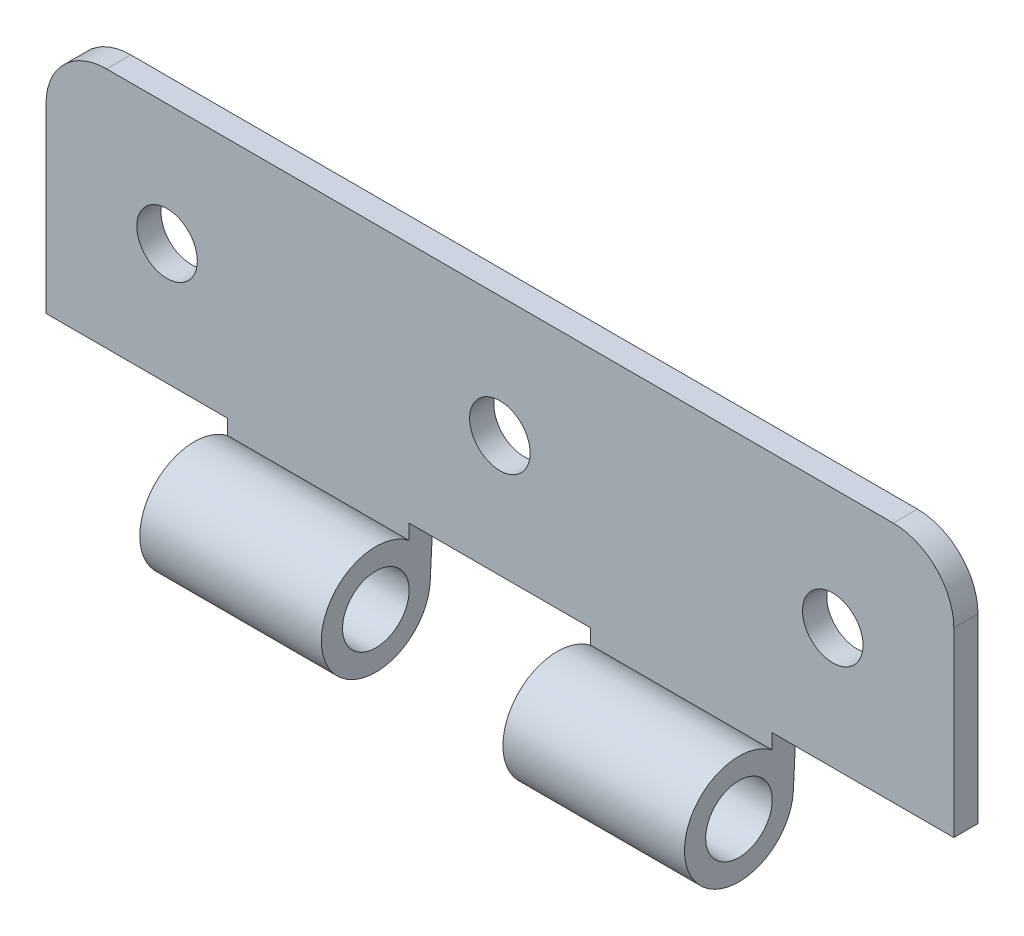
from build123d import *

# Parameters (mm, degrees)
SKETCH1_W           = 75
SKETCH1_H           = 20
SKETCH1_R           = 2.5
BOSS_EXTRUDE1_DEPTH = 2
BOSS_EXTRUDE2_START = -15
BOSS_EXTRUDE2_DEPTH = 15
LPATTERN1_COUNT     = 2
LPATTERN1_PITCH     = 30
FILLET1_R           = 5


with BuildPart() as part:
    # Sketch1 → Boss-Extrude1 (new body)
    with BuildSketch(Plane.XY):
        with Locations((37.5, -10)):
            Rectangle(SKETCH1_W, SKETCH1_H)
        with Locations((10, -10)):
            Circle(SKETCH1_R, mode=Mode.SUBTRACT)
        with Locations((65, -10)):
            Circle(SKETCH1_R, mode=Mode.SUBTRACT)
        with Locations((37.5, -10)):
            Circle(SKETCH1_R, mode=Mode.SUBTRACT)
    extrude(amount=BOSS_EXTRUDE1_DEPTH)

    # Sketch2 → Boss-Extrude2 (add)
    # profile 1 of 2: a face of its own
    with BuildSketch(Plane.ZY.offset(BOSS_EXTRUDE2_START)):
        with BuildLine():
            ThreePointArc((2, -28.361951712), (9.25, -24.8), (2, -21.238048288))
            Line((2, -21.238048288), (2, -24.8))
            Line((2, -24.8), (2, -28.361951712))
        make_face()
        with BuildLine():
            ThreePointArc((7.5, -24.8), (4.75, -27.55), (2, -24.8))
            ThreePointArc((2, -24.8), (4.75, -22.05), (7.5, -24.8))
        make_face(mode=Mode.SUBTRACT)
    # profile 2 of 2: a face of its own
    with BuildSketch(Plane.ZY.offset(BOSS_EXTRUDE2_START)):
        with BuildLine():
            Line((2, -21.238048288), (2, -20))
            Line((2, -20), (0, -20))
            Line((0, -20), (0.255811418, -25.028624118))
            ThreePointArc((0.255811418, -25.028624118), (0.762853744, -26.886304085), (2, -28.361951712))
            Line((2, -28.361951712), (2, -24.8))
            Line((2, -24.8), (2, -21.238048288))
        make_face()
    boss_extrude2 = extrude(amount=-BOSS_EXTRUDE2_DEPTH)

    # LPattern1: Boss-Extrude2 ×2
    with Locations(*[(i * LPATTERN1_PITCH, 0, 0) for i in range(1, LPATTERN1_COUNT)]):
        add(boss_extrude2)

    # Fillet1
    fillet1_edges = [part.edges().sort_by_distance(p)[0] for p in [
        (0, 0, 1),
        (75, 0, 1),
    ]]
    fillet(fillet1_edges, radius=FILLET1_R)


solid = part.part
